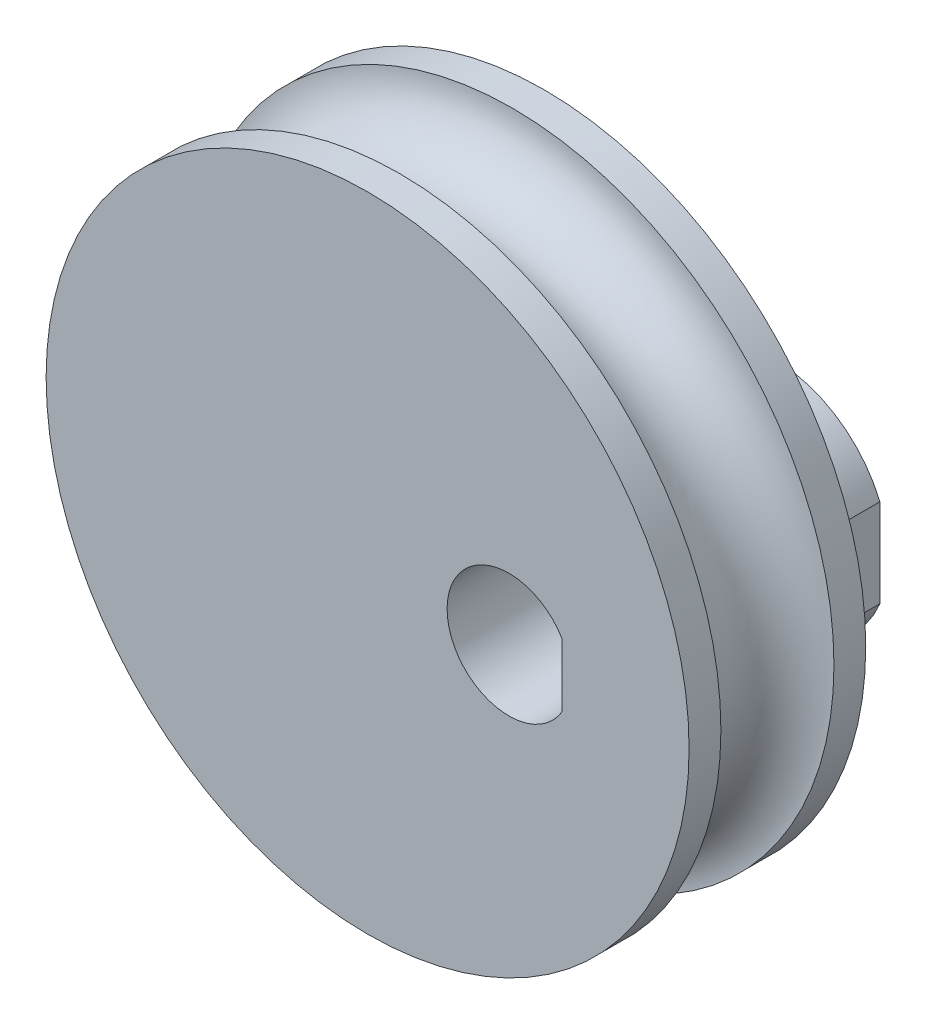
from build123d import *

# Parameters (mm, degrees)
SKETCH_1_R      = 15
EXTRUDE_1_DEPTH = 5
EXTRUDE_2_DEPTH = 5
M3X0_5_1_D      = 2.5
M3X0_5_1_DEPTH  = 7.5
M3X0_5_1_TIP    = 0.751075774


with BuildPart() as part:
    # 草图1 → 凸台-拉伸1 (new, symmetric)
    with BuildSketch(Plane.XY):
        Circle(SKETCH_1_R)
        with BuildLine():
            Line((11, 1.802775638), (11, -1.802775638))
            ThreePointArc((11, -1.802775638), (4.5, 0), (11, 1.802775638))
        make_face(mode=Mode.SUBTRACT)
    extrude(amount=EXTRUDE_1_DEPTH, both=True)

    # 草图4 → 旋转1 (revolve)
    with BuildSketch(Plane(origin=(0, 0, 0), x_dir=(1, 0, 0), z_dir=(0, 1, 0))):
        with BuildLine():
            Line((18.2, 5), (15, 5))
            Line((15, 5), (15, 0))
            ThreePointArc((15, 0), (15.9372583, 2.2627417), (18.2, 3.2))
            Line((18.2, 3.2), (18.2, 5))
        make_face()
        with BuildLine():
            ThreePointArc((18.2, -3.2), (15.9372583, -2.2627417), (15, 0))
            Line((15, 0), (15, -5))
            Line((15, -5), (18.2, -5))
            Line((18.2, -5), (18.2, -3.2))
        make_face()
    revolve(axis=Axis((0, 0, 0), (0, 0, -1)))

    # 草图5 → 凸台-拉伸2 (add)
    with BuildSketch(Plane.XY.offset(-5)):
        with BuildLine():
            Line((14, -2.5), (14, 2.5))
            ThreePointArc((14, 2.5), (1.5, 0), (14, -2.5))
        make_face()
        with BuildLine():
            Line((11, -1.802775638), (11, 1.802775638))
            ThreePointArc((11, 1.802775638), (4.5, 0), (11, -1.802775638))
        make_face(mode=Mode.SUBTRACT)
    extrude(amount=-EXTRUDE_2_DEPTH)

    # M3x0.5 螺纹孔1
    with Locations(Plane(origin=(14, 0, -7.5), x_dir=(0, 0, 1), z_dir=(1, 0, 0))):
        with Locations((0, 0)):
            Hole(M3X0_5_1_D / 2, depth=M3X0_5_1_DEPTH)
            with Locations((0, 0, -(M3X0_5_1_DEPTH + M3X0_5_1_TIP / 2))):  # 118° drill point
                Cone(0, M3X0_5_1_D / 2, M3X0_5_1_TIP, mode=Mode.SUBTRACT)


solid = part.part
